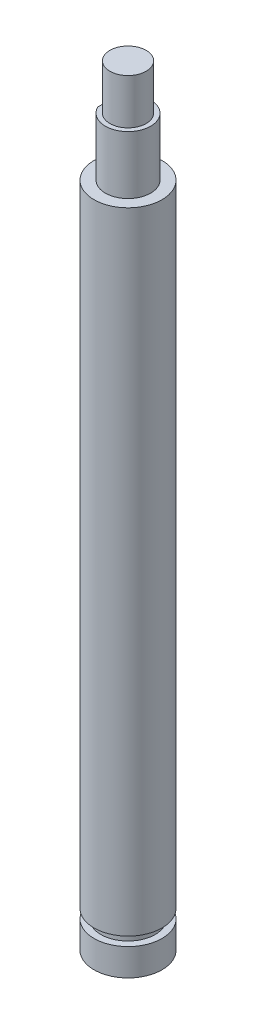
SolidWorks part; units mm, degrees
material "SUS 304"
ref_plane "Front Plane" through (0, 0, 0) normal (0, 0, 1) x (1, 0, 0)
ref_plane "Top Plane" through (0, 0, 0) normal (0, 1, 0) x (1, 0, 0)
ref_plane "Right Plane" through (0, 0, 0) normal (1, 0, 0) x (0, 0, -1)
sketch "Sketch1" plane through (0, 0, 0) normal (0, 0, 1) x (1, 0, 0)
  line L0 (0, 0) -> (7.5, 0)
  line L1 (7.5, 0) -> (7.5, 147.2)
  line L2 (7.5, 147.2) -> (5, 147.2)
  line L3 (5, 147.2) -> (5, 160)
  line L4 (5, 160) -> (4, 160)
  line L5 (4, 160) -> (4, 170)
  line L7 (0, 170) -> (0, 0)
  line L8 (0, -11.2547) -> (0, 0) construction
  line L9 (4, 170) -> (0, 170)
  dimension "D1" = 15
  dimension "D2" = 10
  dimension "D3" = 8
  dimension "D4" = 170
  dimension "D5" = 12.8
  dimension "D6" = 10
revolve "Revolve1" add sketch "Sketch1" angle 360 about L8
sketch "Sketch2" plane through (0, 160, 0) normal (0, 1, 0) x (1, 0, 0)
  line L5 (-4.5, -8.5353) -> (-8.087, -8.5353)
  line L6 (-4.5, -8.5353) -> (-4.5, 6.7634)
  line L7 (-4.5, 6.7634) -> (-8.087, 6.7634)
  line L8 (-8.087, -8.5353) -> (-8.087, 6.7634)
  dimension "D1" = 4.5
extrude "Cut-Extrude1" cut sketch "Sketch2" against normal up to surface (12.8 mm away) up to face at (0, 147.2, -5)
sketch "Sketch3" plane through (0, 0, 0) normal (0, 0, 1) x (1, 0, 0)
  line L0 (0, 0) -> (0, 9.8885) construction
  line L1 (6, 6) -> (10.2756, 6)
  line L2 (6, 6) -> (6, 8)
  line L3 (6, 8) -> (10.2756, 8)
  line L4 (10.2756, 6) -> (10.2756, 8)
  line L5 (-7.5, 0) -> (7.5, 0) construction
  dimension "D1" = 12
  dimension "D2" = 6
  dimension "D3" = 2
revolve "Cut-Revolve1" cut sketch "Sketch3" angle 360 about L0
